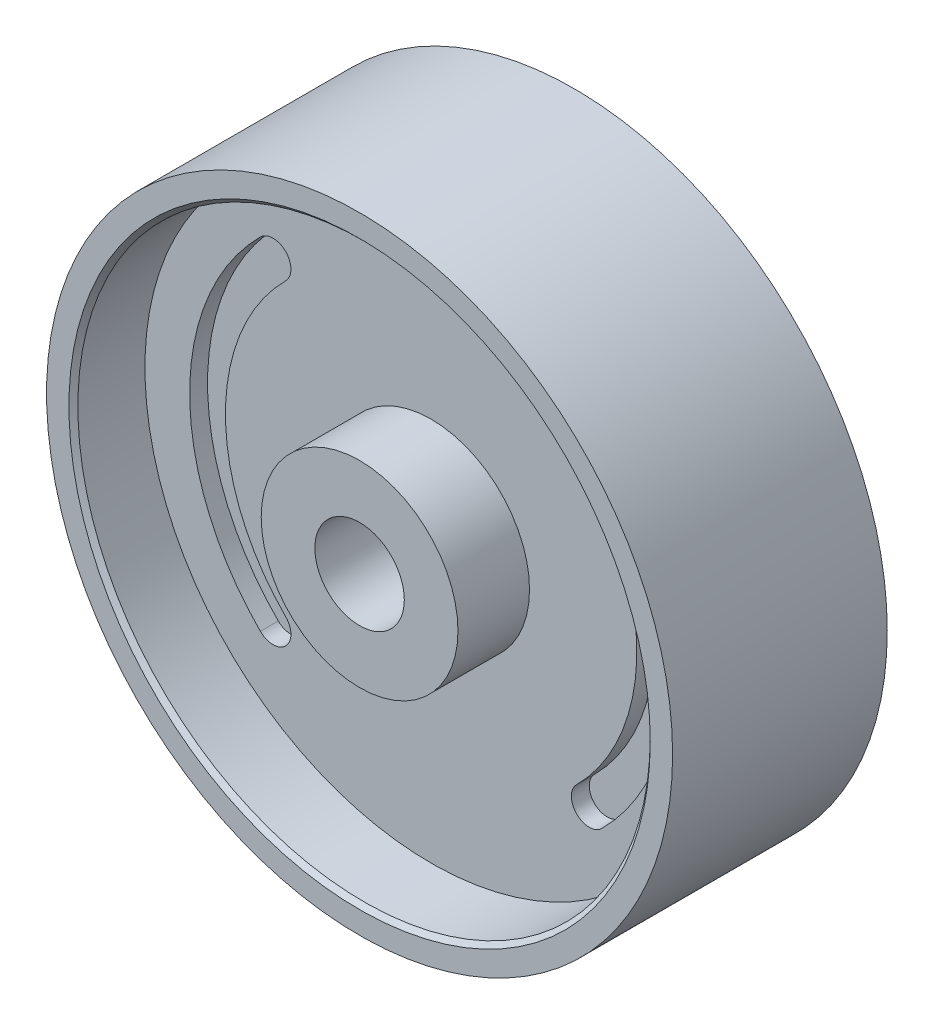
SolidWorks part; units mm, degrees
ref_plane "Front Plane" through (0, 0, 0) normal (0, 0, 1) x (1, 0, 0)
ref_plane "Top Plane" through (0, 0, 0) normal (0, 1, 0) x (1, 0, 0)
ref_plane "Right Plane" through (0, 0, 0) normal (1, 0, 0) x (0, 0, -1)
sketch "Sketch1" plane through (0, 0, 0) normal (0, 0, 1) x (1, 0, 0)
  circle A0 centre (0, 0) radius 35
  dimension "D1" = 70
extrude "Boss-Extrude1" add sketch "Sketch1" along normal mid plane 24
sketch "Sketch2" plane through (0, 0, 12) normal (0, 0, 1) x (1, 0, 0)
  circle A0 centre (0, 0) radius 5
  dimension "D1" = 10
extrude "Cut-Extrude1" cut sketch "Sketch2" against normal mid plane 141
sketch "Sketch3" plane through (0, 0, 12) normal (0, 0, 1) x (1, 0, 0)
  circle A0 centre (0, 0) radius 32
  circle A1 centre (0, 0) radius 11
  dimension "D1" = 64
  dimension "D2" = 22
extrude "Cut-Extrude2" cut sketch "Sketch3" against normal blind 8
mirror "Mirror1" about plane through (0, 0, 0) normal (0, 0, 1) of "Cut-Extrude2"
sketch "Sketch4" plane through (0, 0, -4) normal (0, 0, -1) x (-1, 0, 0)
  line L0 (0, 0) -> (17.6777, 17.6777) construction
  line L1 (0, 0) -> (17.6777, -17.6777) construction
  line L2 (-38.3716, 0) -> (38.3716, 0) construction
  line L3 (0, 0) -> (0, 26.8962) construction
  line L4 (0, 0) -> (-17.6777, -17.6777) construction
  line L5 (0, 0) -> (-17.6777, 17.6777) construction
  arc A0 (17.6777, 17.6777) -> (17.6777, -17.6777) centre (0, 0) cw construction
  arc A1 (19.0919, -19.0919) -> (19.0919, 19.0919) centre (0, 0) ccw
  arc A2 (16.2635, -16.2635) -> (16.2635, 16.2635) centre (0, 0) ccw
  arc A3 (16.2635, -16.2635) -> (19.0919, -19.0919) centre (17.6777, -17.6777) ccw
  arc A4 (19.0919, 19.0919) -> (16.2635, 16.2635) centre (17.6777, 17.6777) ccw
  arc A5 (-17.6777, 17.6777) -> (-17.6777, -17.6777) centre (0, 0) ccw construction
  arc A6 (-19.0919, -19.0919) -> (-19.0919, 19.0919) centre (0, 0) cw
  arc A7 (-16.2635, -16.2635) -> (-16.2635, 16.2635) centre (0, 0) cw
  arc A8 (-16.2635, -16.2635) -> (-19.0919, -19.0919) centre (-17.6777, -17.6777) cw
  arc A9 (-19.0919, 19.0919) -> (-16.2635, 16.2635) centre (-17.6777, 17.6777) cw
  point P3 (25, 0)
  point P18 (-25, 0)
  dimension "D1" = 25
  dimension "D4" = 2
  dimension "D2" = 90
  dimension "D3" = 45
extrude "Cut-Extrude3" cut sketch "Sketch4" against normal blind 2
mirror "Mirror2" about plane through (0, 0, 0) normal (0, 0, 1) of "Cut-Extrude3"
chamfer "Chamfer1" distance 0.5 angle 45 2 edges at (32, 0, -12) (32, 0, 12)
